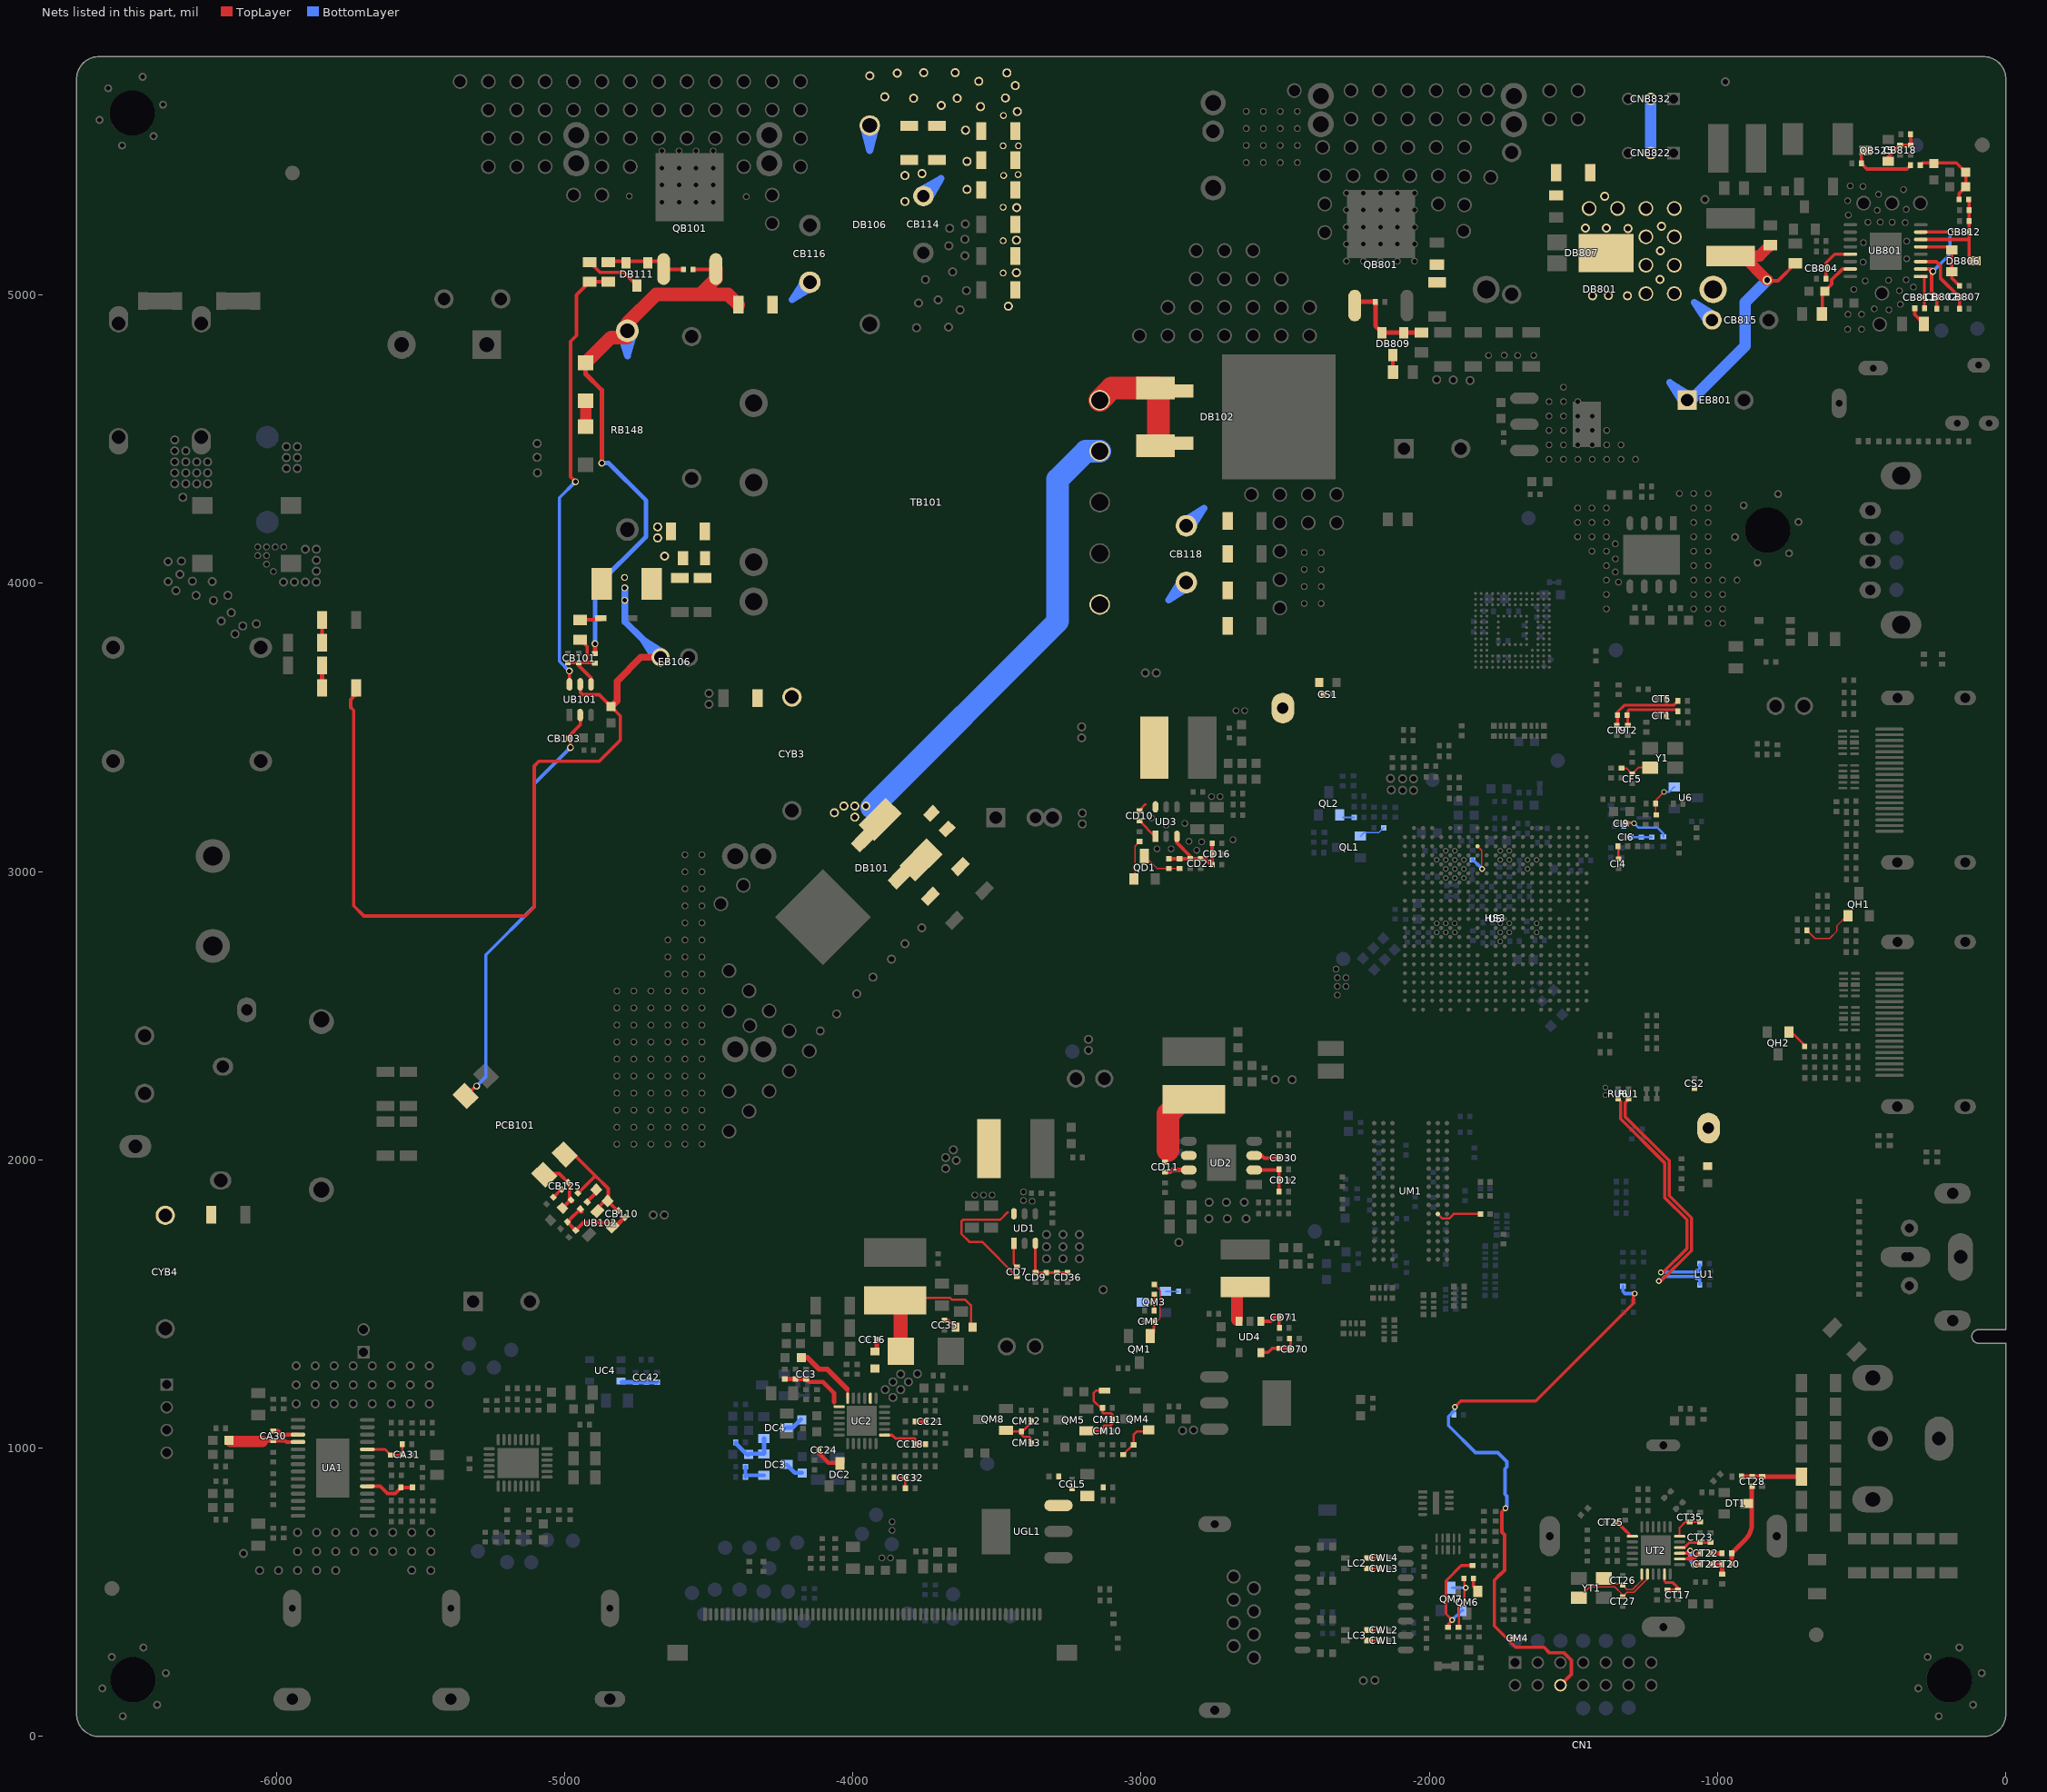
[diagram p0: the nets of this part, all layers, seen from the top]
# Altium PCB MISC84395.PcbDoc (part 21 of 26)
Units mil, origin at the board's own origin, x right, y up, seen from the top; angles counter-clockwise.
Board outline 6692.91 x 5826.77 mil, 2 copper layers (TopLayer, BottomLayer), stack 61.855 mil thick; 951 components, 565 nets, 4374 pads, 1804 vias.
Unrouted connection lines stored in the file: 1.

## Via types
v1: diameter 19.68, hole 11.81, TopLayer to BottomLayer, tented both sides, 1262 vias
v2: diameter 23.62, hole 15.75, TopLayer to BottomLayer, tented both sides, 524 vias
v3: diameter 31.5, hole 19.68, TopLayer to BottomLayer, tented both sides, 11 vias
v4: diameter 24, hole 16, TopLayer to BottomLayer, tented both sides, 6 vias
v5: diameter 19, hole 11.81, TopLayer to BottomLayer, tented both sides, 1 vias

## Nets (pads, with @x,y where several pads share a name; then routed paths per layer and width w, separated by ;. In a path a pad name is that pad's centre, name@x,y a point inside that pad or via, vN(x,y) a via of type N, cw(c..) or ccw(c..) an arc to the next point about the centre after c; other vN are vias at no path point) (continued)
NetCA30_1: CA30.1 LBA4.1 UA1.18 | length 232.8
  TopLayer w13: -6045.8,1026.21 CA30.1@-6010.6,1026.21 -5968.64,1026.21 -5963.94,1021.51 UA1.18@-5924.23,1021.51
  TopLayer w40: LBA4.1@-6157.49,1023.78 -6048.23,1023.78
NetCA30_2: CA30.2 UA1.17 | length 91.6
  TopLayer w13: CA30.2@-6010.6,1059.68 -5994.62,1059.68 -5982.04,1047.1 UA1.17@-5924.23,1047.1
NetCA31_1: CA31.1 RA11.2 RA21.2 UA1.10 | length 173.9
  TopLayer w8: UA1.10@-5684.07,995.92 -5622.59,995.92 RA11.2@-5602.61,975.94 -5558.43,975.94 -5563.33,980.83 RA21.2@-5563.33,1013.94
NetCB101_1: CB101.1 RB103.2 RB105.1 RB121.2 UB101.4 | length 287.9
  TopLayer w11.81: RB103.2@-4988.43,3724.09 CB101.1@-4950.43,3724.09 ; RB121.2@-4956.49,3804.11 -4945.3,3804.11 -4921.49,3780.3 -4921.49,3724.09 ; UB101.4@-4908.09,3649.3 -4908.09,3671.9 -4950.43,3714.24 CB101.1@-4950.43,3724.09 ; RB105.1@-4894.49,3722.83 -4895.74,3724.09 -4921.49,3724.09 ; CB101.1@-4950.43,3724.09 -4921.49,3724.09
NetCB102_1: CB102.1 DB104.K EB106.1 pad.VIA5@-4677,4157.3 pad.VIA5@-4677,4195.3 pad.VIA5@-4791,3941 pad.VIA5@-4791,3984 pad.VIA5@-4792,4020 RB102.1 RB116.1 UB101.5 | length 3115.5
  TopLayer w11.81: RB102.1@-5728.3,3631.59 RB102.1@-5722.89,3637 -5722.89,3610.72 -5726.65,3610.72 -5741.72,3595.65 -5741.72,3569.41 -5731.3,3559 -5731.3,2881.12 -5696.19,2846 -5135.76,2846 -5105.41,2876.35 -5105.41,3366.08 -5089,3382.49 -4879.3,3382.49 -4806.49,3455.3 -4806.49,3539.92 CB102.1@-4838.49,3571.92 -4879.87,3613.3 -4936.49,3613.3 -4945.49,3622.3 UB101.5@-4945.49,3649.3
  TopLayer w23.62: CB102.1@-4838.49,3571.92 -4817.8,3592.61 -4817.8,3660.2 -4735,3743 EB106.1@-4667,3743
  BottomLayer w23.62: pad.VIA5@-4791,3984 pad.VIA5@-4791,3941 -4791,3867 -4728.25,3804.25 EB106.1@-4667,3743
NetCB103_1: CB103.1 PCB101.4 UB101.2 | length 1493
  TopLayer w11.81: PCB101.4@-5342.71,2221.29 -5308,2256 v2(-5305,2256) ; v2(-4979.49,3430.3) -4979.49,3455.3 CB103.1@-4985.49,3461.3 -4985.49,3468.3 -4945.49,3508.3 UB101.2@-4945.49,3543
  BottomLayer w11.81: v2(-5305,2256) -5273.19,2287.81 -5273.19,2711.36 -5105.41,2879.15 -5105.41,3304.38 v2(-4979.49,3430.3)
NetCB109_1: CB109.1 CB110.1 PCB101.2 RB132.1 UB102.K | length 462.1
  TopLayer w11.81: PCB101.2@-4999.18,2019.18 -4968.18,2019.18 -4887,1938 ; RB132.1@-4953.34,1884.66 -4895,1943 -4895,1947 -4848,1900 -4848,1856 -4845.67,1853.67 CB109.1@-4839.67,1853.67 ; UB102.K@-4895,1823 -4860.33,1857.67 CB109.1@-4850.67,1857.67 ; CB109.1@-4845.67,1852.67 -4812.17,1819.17 CB110.1@-4808.17,1819.17
NetCB109_2: CB109.2 RB133.1 | length 55.6
  TopLayer w11.81: RB133.1@-4922.34,1854.66 CB109.2@-4883,1894
NetCB110_2: CB110.2 RB133.2 RB134.2 RB135.2 UB102.R | length 421.9
  TopLayer w11.81: -4980.17,1794.83 RB133.2@-4950,1825 ; RB133.2@-4945,1820 -4940,1825 -4940,1820 ; UB102.R@-4841.97,1769.97 -4835.04,1769.97 UB102.R@-4825.04,1769.97 ; UB102.R@-4823.04,1764.97 -4830.04,1764.97 UB102.R@-4825.04,1769.97 ; CB110.2@-4794.5,1800.5 UB102.R@-4825.04,1769.97 ; CB110.2@-4789.5,1800.5 -4820.04,1769.97 UB102.R@-4825.04,1769.97
  TopLayer w12: RB133.2@-4950,1825 RB135.2@-4990.17,1784.83 RB134.2@-4961.17,1755.83 -4935,1782 -4847.07,1782 UB102.R@-4835.04,1769.97 ; RB133.2@-4945,1820 -4940,1820
NetCB113_1: CB113.1 DB104.A pad.VIA5@-4653,4094.3 RB114.1 RB115.1
NetCB113_2: CB113.2 RB116.2
NetCB114_1: CB114.1@-3755,5343 pad.VIA5@-3760,5421 pad.VIA5@-3819,5324 pad.VIA5@-3819,5414 RB117.1 RB118.1
NetCB116_1: CB116.1 RB119.2
NetCB117_1: CB117.1 DB101.1 DB101.3 pad.VIA5@-3955,3227 pad.VIA5@-3993,3189 pad.VIA5@-3993,3227 pad.VIA5@-4031,3227 pad.VIA5@-4064,3204 TB101.7@-3143.53,3926.18 TB101.10 | length 1590.8
  BottomLayer w78.74: -3934.5,3222.5 -3289,3868 -3289,4360 -3191.32,4457.68 TB101.10@-3143.53,4457.68
NetCB117_2: CB117.2 RB128.1 RB129.1
NetCB118_1: CB118.1 DB102.1 DB102.3 TB101.11 | length 420.5
  TopLayer w78.74: TB101.11@-3143.53,4634.84 -3102.07,4676.3 -2940.17,4676.3 DB102.3@-2940.17,4476.3
NetCB118_2: CB118.2 RB124.1 RB125.1 RB126.1 RB136.1
NetCB125_1: CB125.1 PCB101.1 RB131.1 RB132.2 | length 212.2
  TopLayer w11.81: PCB101.1@-5072.89,1952.47 -5018.51,1952.47 -4983,1916.96 -4983,1865 RB132.2@-4979,1861 ; RB131.1@-5006.94,1833.06 RB132.2@-4979,1861 ; RB132.2@-4975,1857 RB132.2@-4974,1856 ; RB132.2@-4972,1856 RB132.2@-4974,1856 ; RB132.2@-4979,1861 RB132.2@-4974,1856
NetCB125_2: CB125.2 RB158.1 | length 39.4
  TopLayer w11.81: RB158.1@-5039.12,1869.99 CB125.2@-5011.24,1897.87
NetCB802_2: CB802.2 RB802.2 UB801.2 UB801.7 | length 441.7
  TopLayer w11.81: UB801.2@-295.53,5089.88 v2@-255.2,5089.88 ; UB801.7@-295.53,5217.83 -295.36,5218 v2(-194,5218) ; v2(-253.19,5081.87) -258,5077.05 -258,5010.59 CB802.2@-239.73,4992.32 RB802.2@-239.73,4952.32
  BottomLayer w11.81: v2(-253.19,5081.87) -194,5141.05 v2(-194,5218)
NetCB804_2: CB804.2 RB805.2 UB801.13 | length 150.5
  TopLayer w9.84: RB805.2@-624,5056 CB804.2@-624,5085.94 ; CB804.2@-620.03,5091.94 CB804.2@-624,5091.94 -624,5110.98 -593.92,5141.06 UB801.13@-539.63,5141.06 UB801.13@-540.17,5141.6
NetCB805_2: CB805.2 RB804.1 | length 67.2
  TopLayer w11.81: RB804.1@-316.2,4953.32 -316.2,4931.24 CB805.2@-284.27,4899.32
NetCB807_1: CB807.1 RB801.2 UB801.3 | length 250.5
  TopLayer w11.81: UB801.3@-295.53,5115.47 -241.47,5115.47 -227.47,5101.47 -227.47,5058.79 CB807.1@-161,4992.32 RB801.2@-161,4952.32
NetCB809_1: CB809.1 RB810.1
NetCB810_1: CB810.1 RB811.1
NetCB811_1: CB811.1 RB804.2 UB801.1 | length 123.8
  TopLayer w9.84: UB801.1@-295.53,5064.29 -282.73,5064.29 RB804.2@-282.73,4953.32
NetCB812_2: CB812.2 DB806.2 RB812.2 RB822.2 RB837.2 UB801.6 | length 382.6
  TopLayer w11.81: UB801.6@-295.53,5192.24 -128.71,5192.24 -127.95,5193 ; RB837.2@-127.95,5322.27 RB822.2@-127.95,5294.13 RB812.2@-127.95,5256.13 CB812.2@-127.95,5218 -127.95,5193 ; DB806.2@-109.97,5115 -127.95,5132.98 -127.95,5193
NetCB813_2: CB813.2 RB816.1 UB801.15 | length 212.9
  TopLayer w11.81: RB816.1@-644.19,4916.79 -637,4923.98 -637,4997 ; CB813.2@-628.19,5013 -604.24,5036.95 -604.24,5047 -604.24,5052.76 -567.12,5089.88 UB801.15@-539.63,5089.88
NetCB814_1: CB814.1 CB816.1 CB819.1 RB830.1 RB837.1 | length 279
  TopLayer w11.81: RB830.1@-297.27,5450 -289.27,5458 -172,5458 CB814.1@-139,5425 CB816.1@-139,5375 -162.46,5351.54 RB837.1@-162.46,5331
NetCB815_1: CB815.1 DB801.K DB807.2 EB801.1@-1105.65,4635 LB804.1 pad.VIA5@-828,5051 pad.VIA5@-1150.45,5004.44 pad.VIA5@-1150.45,5102.87 pad.VIA5@-1150.45,5201.29 pad.VIA5@-1150.45,5299.72 pad.VIA5@-1194.89,5238 pad.VIA5@-1198.89,5153 pad.VIA5@-1199.89,5054 pad.VIA5@-1248.88,5004.44 pad.VIA5@-1248.88,5102.87 pad.VIA5@-1248.88,5201.29 pad.VIA5@-1248.88,5299.72 pad.VIA5@-1310.89,5230 pad.VIA5@-1312.89,4997 pad.VIA5@-1347.3,5299.72 pad.VIA5@-1378.89,4998 pad.VIA5@-1385.89,5232 pad.VIA5@-1391.89,5342 pad.VIA5@-1433.89,4997 pad.VIA5@-1445.73,5299.72 pad.VIA5@-1458.89,5232 RB811.2 RB814.2 RB824.1 | length 984.6
  TopLayer w3: RB814.2@-747,5108 -745.09,5109.91 RB814.2@-730,5109.91
  TopLayer w11.81: pad.VIA5@-826.57,5049 -790.91,5049 RB814.2@-730,5109.91
  TopLayer w39.37: pad.VIA5@-828,5051 -912.04,5135.04 LB804.1@-955,5135.04 -854.87,5135.04 RB824.1@-823.45,5166.45
  BottomLayer w39.37: EB801.1@-1105.65,4635 -1092.65,4635 -905,4822.65 -905,4974 pad.VIA5@-828,5051
NetCB818_2: CB818.2 QB525.B RB833.1 RB834.2 | length 145.3
  TopLayer w11.81: QB525.B@-409,5463.5 -409,5477.66 -367.66,5519 CB818.2@-367,5519 RB833.1@-330,5519 RB834.2@-330,5554
NetCC3_1: CC3.1 RC7.1 RC9.1 UC2.1 | length 225.1
  TopLayer w15: RC9.1@-4236.24,1240.11 RC7.1@-4199.24,1240.11 CC3.1@-4162.24,1240.11 ; CC3.1@-4161.11,1240.11 CC3.1@-4162.24,1240.11 ; -4065.34,1159 -4065.34,1192.34 -4103,1230 -4152.13,1230 CC3.1@-4162.24,1240.11
NetCC11_1: CC11.1 UC2.24 | length 250.6
  TopLayer w10: -4019.61,1207.61 -4017.95,1205.95 UC2.24@-4017.95,1173.66
  TopLayer w18: CC11.1@-4179,1314 CC11.1@-4166.76,1314 ; CC11.1@-4178,1317 -4169.76,1317 CC11.1@-4166.76,1314 ; -4020.27,1205.95 -4088.32,1274 -4117.23,1274 -4157.23,1314 CC11.1@-4166.76,1314
NetCC16_2: CC16.2 RC11.1 | length 47
  TopLayer w15: RC11.1@-3923,1335.78 RC11.1@-3923,1341.52 ; RC11.1@-3917.26,1341.52 CC16.2@-3917.26,1377 CC16.2@-3917.26,1371.27
NetCC18_2: CC18.2 RC14.1 UC2.13 | length 165.5
  TopLayer w10: UC2.13@-3890,1045.71 -3863.71,1045.71 -3852.16,1034.16 -3787.16,1034.16 -3784.27,1031.27 CC18.2@-3784.27,1014 RC14.1@-3747.73,1014
NetCC21_1: CC21.1 RC13.2 | length 36.5
  TopLayer w10: RC13.2@-3784.26,1093 CC21.1@-3747.73,1093
NetCC24_2: CC24.2 DC2.2 | length 95.7
  TopLayer w15: CC24.2@-4117.57,994 -4117.57,982.57 -4084.5,949.5 -4050.47,949.5 DC2.2@-4048,947.03
NetCC27_1: CC27.1 DC3.2 | length 65.9
  BottomLayer w15: DC3.2@-4229.97,943.19 -4201.16,914.38 CC27.1@-4176,914.38
NetCC28_1: CC28.1 DC3.3 DC4.1 RC23.1 | length 170.9
  BottomLayer w15: RC23.1@-4405.73,1020.19 -4405.73,1017.28 -4366.65,978.19 CC28.1@-4361.19,978.19 -4358.69,980.69 DC3.3@-4308,980.69 DC4.1@-4308,1033.69
NetCC31_1: CC31.1 DC4.2 | length 62.3
  BottomLayer w15: DC4.2@-4229.97,1071.19 -4209.81,1071.19 CC31.1@-4180,1101
NetCC32_1: CC32.1 RC25.1 RC29.2 | length 74.5
  TopLayer w8: RC29.2@-3855.27,898 CC32.1@-3817.73,898 RC25.1@-3817.73,861
NetCC35_2: CC35.2 RC28.1 | length 48.1
  TopLayer w8: CC35.2@-3682,1443.74 -3667.52,1443.74 RC28.1@-3643.78,1420
NetCC42_1: CC42.1 RC31.2 RC35.1 UC4.3 | length 122.5
  BottomLayer w15: UC4.3@-4801.54,1229 RC35.1@-4753,1229 RC31.2@-4679,1229
NetCD7_1: CD7.1 UD1.1 | length 86.4
  TopLayer w8: UD1.1@-3441.4,1710.82 -3441.4,1639.13 CD7.1@-3431,1628.73
NetCD7_2: CD7.2 LD1.1 UD1.6 | length 471.5
  TopLayer w8: -3463,1818 -3489.12,1791.88 -3617.88,1791.88 -3623.46,1786.3 -3623.46,1743.59 -3595.63,1715.75 -3551.35,1715.75 -3431,1595.39 CD7.2@-3431,1595.26 ; UD1.6@-3442.58,1813.18 UD1.6@-3441.4,1813.18
NetCD9_1: CD9.1 CD36.1 RD1.1 RD4.2 UD1.3 | length 212.2
  TopLayer w10: CD9.1@-3366.6,1609.6 UD1.3@-3366.6,1710.82 ; CD9.1@-3366,1609 CD36.1@-3255,1609
NetCD10_1: CD10.1 UD3.1 | length 78
  TopLayer w8: CD10.1@-3005,3176.61 -3005,3175.19 -2951.82,3122.01 UD3.1@-2950.4,3122.01
NetCD10_2: CD10.2 LD3.1 UD3.6 | length 31.2
  TopLayer w8: CD10.2@-3005,3210.07 -3005,3213 -2985,3233
NetCD11_1: CD11.1 LD2.1 UD2.6 | length 197.2
  TopLayer w80: -2906.94,2034.06 -2906.94,2159.06 LD2.1@-2855.87,2210.13
NetCD11_2: CD11.2 UD2.7 | length 85.4
  TopLayer w15: CD11.2@-2917,1958.27 -2899,1958.27 -2892.27,1965 UD2.7@-2834.39,1965
NetCD12_1: CD12.1 RD7.1 RD12.1 UD2.2 | length 160.9
  TopLayer w12: UD2.2@-2607.61,1965 RD7.1@-2523.73,1965 ; RD12.1@-2521.73,1890 CD12.1@-2521.73,1929 RD7.1@-2521.73,1967
NetCD16_1: CD16.1 CD21.1 RD8.1 RD13.2 RD15.2 RD16.2 RD17.2 UD3.3 | length 328.2
  TopLayer w12: RD13.2@-2903.26,3044.57 RD17.2@-2866.26,3044.57 RD16.2@-2829.26,3044.57 ; UD3.3@-2875.6,3122.01 -2875.6,3099.6 -2829.26,3053.26 RD16.2@-2829.26,3044.57 ; RD16.2@-2829.26,3044.44 RD16.2@-2829.26,3044.57 ; CD21.1@-2793.39,3044.57 RD16.2@-2829.26,3044.57 ; CD21.1@-2793.26,3044.44 -2777.44,3044.44 -2757.19,3024.19 RD15.2@-2753.73,3024.19 RD8.1@-2753.73,3097.84
NetCD30_1: CD30.1 UD2.3 | length 89.6
  TopLayer w12: UD2.3@-2607.61,2015 -2582,2015 -2573,2006 CD30.1@-2521.73,2006
NetCD70_1: CD70.1 RD50.1 RD51.2 UD4.5 | length 141.3
  TopLayer w10: UD4.5@-2584.81,1332.15 -2559.85,1332.15 -2545.73,1346.27 RD51.2@-2520,1346.27 -2484.47,1346.27 -2481.73,1349.01 RD50.1@-2481.73,1380.26
NetCD71_2: CD71.2 RD3.1 UD4.1 | length 105.1
  TopLayer w12: UD4.1@-2584.81,1440.42 -2549.84,1440.42 -2536,1454.26 CD71.2@-2521.46,1454.26 RD3.1@-2521.46,1418.26
NetCF5_1: CF5.1 RF1.1 Y1.1 | length 116.5
  TopLayer w6: RF1.1@-1333.65,3358.47 -1316.65,3358.47 CF5.1@-1296.64,3338.47 -1274.38,3360.74 Y1.1@-1234.65,3360.74
NetCGL4_2: CGL4.2 CGL5.1 RG01.1 RG02.1 UGL1.3
NetCI4_2: CI4.2 RI4.1 | length 36.5
  TopLayer w8: CI4.2@-1343.65,3043.48 RI4.1@-1343.65,3080.01
NetCI6_1: CI6.1 RI7.1 RI9.1 | length 72.4
  BottomLayer w8: CI6.1@-1300.92,3119.74 -1264.91,3119.74 RI9.1@-1264.65,3119.47 RI7.1@-1228.65,3119.47
NetCI9_1: CI9.1 RI11.1 RI12.1 | length 184.1
  TopLayer w8: CI9.1@-1315.77,3167.74 v1(-1289.77,3167.74)
  BottomLayer w8: RI12.1@-1324.91,3159.74 -1316.91,3167.74 v1@-1297.65,3167.74 ; v1(-1289.77,3167.74) -1273.77,3151.74 -1208.26,3151.74 -1188.65,3132.13 RI11.1@-1188.65,3120.47
NetCM1_2: CM1.2 QM1.G RM5.2 | length 206.3
  TopLayer w5: CM1.2@-2955.26,1440 -2945,1440 -2935,1450 -2935,1548.73 RM5.2@-2954,1567.73
  TopLayer w8: QM1.G@-2968.6,1389.24 QM1.G@-2964.26,1393.58
  TopLayer w10: QM1.G@-2964.26,1393.58 -2955.26,1402.58 CM1.2@-2955.26,1440
NetCM4_2: CM4.2 CN1.6 RM13.1 RM14.1 | length 2204.5
  TopLayer w11.3: v1(-1912,1143) -1891.51,1163.49 -1631.53,1163.49 -1292.02,1503 v1@-1292.02,1532.42
  TopLayer w12: v1@-1739.17,788.57 -1748.29,779.45 -1748.29,708.71 -1739.17,699.59 -1739.17,576.69 -1753.58,562.28 -1754.72,562.28 -1774.75,542.25 -1774.75,383.85 -1700.3,309.39 -1602.21,309.39 -1583.21,290.39 -1532.75,290.39 -1507,264.64 -1507,216.28 CN1.6@-1545.28,178
  BottomLayer w12: v1(-1912,1143) -1912,1131.84 -1933.84,1110 -1933.84,1078.37 -1840.48,985 -1763,985 -1731.16,953.16 -1731.16,935.37 -1737.84,928.68 -1737.84,840.61 -1731.16,833.92 -1731.16,796.58 v1(-1735.88,791.85) ; RM13.1@-1328.77,1561.54 -1328.77,1543.77 -1321.61,1536.61 v1(-1287.83,1536.61)
NetCM10_2: CM10.2 CM11.1 DM1.K QM5.G RM12.2 | length 300.6
  TopLayer w8: CM10.2@-3133.73,1060 -3133.73,1072.27 -3127,1079 -3106,1079 -3100.27,1084.73 -3100.27,1117.43 -3104,1121.16 -3131.16,1121.16 -3133.73,1123.73 RM12.2@-3133.73,1140 -3140,1140 -3165,1165 -3165,1191 -3156,1200 DM1.K@-3127.15,1200
  TopLayer w10: QM5.G@-3189.16,1060 CM10.2@-3133.73,1060
NetCM12_1: CM12.1 CM13.2 QM8.G RM15.2 | length 167.5
  TopLayer w8: QM8.G@-3464.16,1058 RM15.2@-3414.73,1058 ; CM13.2@-3381.27,1017 -3381.27,1032.27 -3388,1039 -3407,1039 -3414.73,1046.73 RM15.2@-3414.73,1058 ; CM12.1@-3381.27,1095 -3381.27,1089.42 -3412.7,1058 RM15.2@-3414.73,1058
NetCNB822_2: CNB822.2 CNB832.2 | length 188.1
  BottomLayer w39.37: CNB832.2@-1232,5680 -1231.74,5679.74 CNB822.2@-1231.74,5492
NetCS1_1: CS1.1 HS3.1 RS1.2
NetCS2_1: CS2.1 HS3.2@-1031.98,2110.2 RS2.1
NetCT1_1: CT1.1 CT2.1 RT4.2 RT14.2 | length 250
  TopLayer w10: CT2.1@-1311.64,3506.47 -1311.65,3556.35 -1306.26,3561.74 -1143.2,3561.74 RT4.2@-1137.46,3556 ; CT1.1@-1177.43,3540 -1177.43,3561.32
NetCT5_2: CT5.2 CT9.1 RT2.2 RT14.1 | length 290.5
  TopLayer w10: CT9.1@-1347.38,3508.74 RT14.1@-1347.38,3542.74 -1347.38,3553.62 -1324.26,3576.74 -1153.12,3576.74 RT2.2@-1137.73,3592.13 ; -1177.26,3578 CT5.2@-1177.26,3598
NetCT17_2: CT17.2 RT1.1 UT2.23 | length 124.9
  TopLayer w10: UT2.23@-1184.36,563.58 -1184.36,539 -1179.26,533.9 -1155.15,533.9 -1138.21,516.96 CT17.2@-1138.21,507.93 ; RT1.1@-1174.21,507.92 CT17.2@-1138.21,507.93
NetCT20_1: CT20.1 CT28.1 DT1.2 LT6.2 | length 295.6
  TopLayer w15.8: CT20.1@-951.27,598.68 ccw(c-950.94,598.68) -951.17,598.45 LT6.2@-951.17,635.76 ccw(c-951.51,635.76) -951.27,636 -903.92,683.35 ccw(c-956.82,736.26) -882,736.26 CT28.1@-882,868.27
NetCT20_2: CT20.2 CT21.1 LT5.2 | length 74.8
  TopLayer w15.8: CT21.1@-1024.27,597.68 CT20.2@-984.74,597.69 -984,596.95 LT5.2@-984,562.74
NetCT21_2: CT21.2 UT2.3 | length 131.3
  TopLayer w10: UT2.3@-1113,635.63 UT2.3@-1132,635.63 -1104.37,635.63
  TopLayer w15.8: -1104.37,638.54 -1101.46,638.54 v1(-1095,645) ; v1(-1083,595) -1060.42,595 CT21.2@-1057.74,597.69
  BottomLayer w15.8: v1@-1095,641 -1095,626.97 ccw(c-1054.03,626.97) v1@-1083,598
NetCT22_1: CT22.1 LT6.1 | length 40
  TopLayer w15.8: CT22.1@-1024.68,635.76 LT6.1@-984.64,635.76
NetCT22_2: CT22.2 UT2.2 | length 77
  TopLayer w10: UT2.2@-1132,615.94 -1103.29,615.94
  TopLayer w15.8: -1100.39,617.73 -1096.96,617.73 ccw(c-1096.96,650.77) -1073.59,627.41 -1065.27,635.73 CT22.2@-1058.17,635.73
NetCT23_1: CT23.1 LT1.2 UT2.4 | length 120.1
  TopLayer w10: UT2.4@-1132,655.32 -1115.74,655.32 -1097.79,673.26 LT1.2@-1024.28,673.26 LT1.2@-1019.28,673.26
NetCT25_2: CT25.2 UT2.13 | length 80.7
  TopLayer w10: -1316.41,711.37 -1299.72,694.69 UT2.13@-1295.78,694.69
  TopLayer w12: CT25.2@-1355.27,746 -1351.03,746 -1316.41,711.37
NetCT26_2: CT26.2 UT2.19 YT1.1 | length 159.3
  TopLayer w5: YT1.1@-1378.29,529.31 CT26.2@-1330.28,529.31 ; CT26.2@-1329.28,529.31 CT26.2@-1329.28,525.26 -1314.02,510 -1295.19,510 -1263.1,542.09 UT2.19@-1263.1,563.58
NetCT27_2: CT27.2 UT2.20 YT1.3 | length 313.7
  TopLayer w5: YT1.3@-1481.31,481.54 -1443.53,519.31 -1357.31,519.31 -1329.29,491.29 CT27.2@-1329.29,484.74 -1314.03,500 -1291.05,500 -1243.42,547.63 UT2.20@-1243.42,563.58
NetCT28_2: CT28.2 CT60.2 DT4.K LT2.1 | length 209.9
  TopLayer w15.8: LT2.1@-917,901.15 -724.04,901.15 ccw(c-724.04,922.67) CT60.2@-708.82,907.46
NetCT35_1: CT35.1 RT6.1 UT2.6 | length 110.9
  TopLayer w5: RT6.1@-1061,744.27 -1059.91,744.27 RT6.1@-1059.12,743.49
  TopLayer w7: UT2.6@-1132,694.69 -1132,724 -1111.73,744.27 CT35.1@-1097,744.27 RT6.1@-1061,744.27
NetCWL1_2: CWL1.2 LC3.2 | length 37.4
  TopLayer w7: LC3.2@-2209.12,333 CWL1.2@-2171.74,333
NetCWL2_2: CWL2.2 LC3.3 | length 37.4
  TopLayer w7: LC3.3@-2209.13,369 CWL2.2@-2171.73,369
NetCWL3_2: CWL3.2 LC2.2 | length 41.7
  TopLayer w7: LC2.2@-2211.12,583 CWL3.2@-2173.73,583 ; LC2.2@-2201.24,582.88 LC2.2@-2196.88,582.88
NetCWL4_2: CWL4.2 LC2.3 | length 39
  TopLayer w7: LC2.3@-2210.35,620 CWL4.2@-2173.73,620 ; LC2.3@-2201.24,619.11 LC2.3@-2198.89,619.11
NetCYB3_1: CYB3.1 RB130.2
NetCYB4_1: CYB4.1 RB5.1
NetD4_K: D4.K R21.2 U6.2 | length 137.5
  TopLayer w6: R21.2@-1215.04,3197.01 D4.K@-1215.04,3235.74 ; D4.K@-1211.77,3235.74 D4.K@-1215.04,3235.74 ; v1(-1186,3276) -1200.68,3261.32 -1215.04,3246.96 D4.K@-1215.04,3235.74
  BottomLayer w6: v1(-1186,3276) -1167.5,3276 U6.2@-1150,3293.5
NetDB106_K: DB106.K pad.VIA5@-3557,5653 pad.VIA5@-3563,5741 pad.VIA5@-3604,5366 pad.VIA5@-3604,5463 pad.VIA5@-3609,5571 pad.VIA5@-3638,5682 pad.VIA5@-3645,5771 pad.VIA5@-3693,5657 pad.VIA5@-3754,5771 pad.VIA5@-3789,5682 pad.VIA5@-3846,5769 pad.VIA5@-3889,5687 pad.VIA5@-3941,5760 RB117.2 RB118.2 RB151.1 RB154.1 RB155.1
NetDB109_A: DB109.A QB101.S RB105.2 RB109.1 RB119.1 RB148.2 | length 2026.9
  TopLayer w11.81: RB109.1@-4554.54,5088 QB101.S@-4493.39,5088
  TopLayer w15.75: DB109.A@-4927,4764.74 -4927,4726 -4871,4670 v2(-4871,4417) ; RB105.2@-4894.49,3756.3 -4894,3756.79 v2(-4894,3790)
  TopLayer w47.24: DB109.A@-4927,4764.74 -4839.51,4852.23 -4782,4852.23 RB148.2@-4782,4875.23 -4782,4902 -4683,5001 -4432,5001 RB119.1@-4397,4966 ; -4530,5001 -4475.16,5055.84 QB101.S@-4475.16,5089.54
  BottomLayer w15.75: v2(-4894,3790) -4894,3985 -4717,4162 -4717,4287 -4847,4417 v2(-4871,4417)
NetDB109_K: DB109.K DB110.A | length 90.1
  TopLayer w39.37: DB110.A@-4927,4542.74 DB109.K@-4927,4632.85
NetDB111_1: DB111.1 DB111.3 QB101.G RB106.2 RB109.2 | length 280.5
  TopLayer w11.81: RB106.2@-4847.47,5117 QB101.G@-4656.26,5117 ; QB101.G@-4656.26,5065.98 QB101.G@-4656.26,5093.98 ; QB101.G@-4656.26,5066.09 QB101.G@-4656.15,5065.98 ; QB101.G@-4649.15,5088 RB109.2@-4588,5088
NetDB111_2: DB111.2 RB107.2 | length 197.3
  TopLayer w11.81: RB107.2@-4912.57,5113.87 -4876.7,5078 -4794.4,5078 DB111.2@-4748.97,5032.57
NetDB121_K: DB121.K RB121.1 | length 72.6
  TopLayer w11.81: RB121.1@-4946.39,3872.3 RB121.1@-4946.49,3872.39 -4945.88,3873 DB121.K@-4874.3,3873
NetDB806_1: DB806.1 DB806.3 RB827.2 UB801.5 | length 254
  TopLayer w11.81: UB801.5@-295.53,5166.65 -188,5166.65 -188,5058.32 RB827.2@-161,5031.32
NetDB809_1: DB809.1 DB809.3 QB801.G RB807.2 RB808.1 | length 316.7
  TopLayer w15.75: QB801.G@-2258.84,4963 QB801.G@-2255,4959.16 ; QB801.G@-2245.84,4976 RB808.1@-2187.2,4976 -2187.2,4892.2 DB809.3@-2164,4869 -2163.91,4869.09 RB807.2@-2028,4869.09
NetDB809_2: DB809.2 RB809.2 | length 59.2
  TopLayer w11.81: DB809.2@-2126.5,4790.97 -2126.5,4732.5 RB809.2@-2126,4732
NetDC1_A: DC1.A LC1.2 RC11.2 RC28.2 UC2.20 | length 468.1
  TopLayer w8: LC1.2@-3844.44,1521.69 -3662.67,1521.69 -3655.98,1515 -3609.95,1515 -3590.39,1495.44 -3590.39,1426.17 RC28.2@-3584.22,1420
  TopLayer w50: DC1.A@-3834.01,1352 LC1.2@-3834.01,1477.13
NetDC3_1: DC3.1 RC19.1 RC20.2 | length 102.5
  BottomLayer w12: RC20.2@-4372.27,936.19 RC19.1@-4372.27,900.19 -4366.77,905.69 DC3.1@-4308,905.69
NetLD5_1: LD5.1 UD4.3 | length 125.7
  TopLayer w40: UD4.3@-2667.21,1445.26 -2667.21,1531.09 LD5.1@-2639,1559.3
NetLU1_2: LU1.2 RU6.1 RU8.2 | length 896.3
  TopLayer w11: RU6.1@-1344.83,2210.23 -1336.83,2202.23 -1336.83,2142.66 -1184.34,1990.17 -1184.34,1869.37 -1107,1792.03 -1107,1692.49 -1189.6,1609.88 v1(-1196.74,1609.88)
  BottomLayer w11: v1(-1196.74,1609.88) -1195.86,1609 -1193.86,1611 -1080,1611 -1076.19,1614.81 LU1.2@-1067.65,1614.81 -1062.73,1619.73 RU8.2@-1062.73,1637
NetLU1_3: LU1.3 RU1.1 RU2.2 | length 940.3
  TopLayer w11: RU1.1@-1308.83,2210.23 -1320.83,2198.23 -1320.83,2149.28 -1168.34,1996.79 -1168.34,1876 -1091,1798.65 -1091,1685.86 v1@-1195.26,1581.61
  BottomLayer w11: v1(-1204,1580) -1197.86,1580 -1182.86,1595 -1080,1595 -1076.19,1591.19 LU1.3@-1067.65,1591.19 -1062.73,1586.27 RU2.2@-1062.73,1569
NetMR313_2: MR313.2 UM1.L8 | length 154.5
  TopLayer w7.87: UM1.L8@-1970.75,1812.46 -1955.01,1796.71 -1931.39,1796.71 -1915.64,1812.46 MR313.2@-1829.34,1812.46
NetQB525_C: QB525.C RB830.2 RB832.2 | length 235.3
  TopLayer w11.81: QB525.C@-487.03,5501.5 -501.27,5487.26 RB832.2@-501.27,5456 -482.11,5436.85 -343.89,5436.85 RB830.2@-330.73,5450
NetQD1_D: QD1.D RD13.1 RD17.1 | length 139.6
  TopLayer w5: QD1.D@-2988,3054.19 -2944.91,3011.1 RD13.1@-2903.26,3011.1 RD17.1@-2866.26,3011.1
NetQD1_G: QD1.G RD24.1 | length 138.6
  TopLayer w5: QD1.G@-3025.5,2974.19 -3021.25,2978.44 -3021.25,3088.02 RD24.1@-3005,3104.27
NetQH1_B: QH1.B RH3.1 | length 197.2
  TopLayer w5: RH3.1@-690.1,2796 -662.1,2768 -611.5,2768 -585.83,2793.67 -585.83,2812.63 -551.46,2847 QH1.B@-548.33,2847
NetQH2_B: QH2.B RH12.1 | length 74.2
  TopLayer w7: QH2.B@-752.5,2444.03 -744.73,2444.03 RH12.1@-697.73,2397.03
NetQL1_B: QL1.B RL7.1 | length 93
  BottomLayer w5: QL1.B@-2239,3122.5 -2226.84,3134.66 -2175.61,3134.66 RL7.1@-2158.27,3152
NetQL2_B: QL2.B RL9.1 | length 40.8
  BottomLayer w5: QL2.B@-2301.5,3188 RL9.1@-2260.73,3188
NetQM3_B: QM3.B RM7.2 | length 45
  BottomLayer w5: QM3.B@-2914.97,1544 RM7.2@-2870,1544
NetQM3_C: QM3.C RM1.1 RM5.1 | length 94.3
  TopLayer w5: RM1.1@-2954,1478 v1(-2954,1505) RM5.1@-2954,1534.27
  BottomLayer w5: QM3.C@-2992,1505 v1(-2954,1505)
NetQM4_B: QM4.B RM8.2 RM9.1 | length 144.8
  TopLayer w8: RM9.1@-3062,978.27 -3028.54,1011.73 RM8.2@-3026,1011.73 -3026,1046.75 -3015,1057.75 -2978.75,1057.75 QM4.B@-2973,1063.5
NetQM6_B: QM6.B RK7.1 | length 50.5
  TopLayer w10: RK7.1@-1847.27,548 -1847.27,519.77 QM6.B@-1831.5,504
NetQM7_B: QM7.B RK6.1 RK8.2 | length 343.2
  TopLayer w10: RK6.1@-1935,378.73 -1935,389 -1921,403 v1(-1921,404) -1942.5,425.5 -1942.5,540.07 -1889.3,593.27 RK8.2@-1850,593.27
  BottomLayer w10: v1(-1921,404) -1887,438 QM7.B@-1882.5,438
NetQM7_C: QM7.C RK3.1 RK7.2 | length 224.4
  TopLayer w8: RK3.1@-1898,378.73 -1898,449 -1879,468 -1879,546.27 RK7.2@-1880.73,548
  BottomLayer w8: QM7.C@-1920.5,516.03 v1@-1874.03,516.03
  other v1: -1874,516
NetR50_1: R50.1 U5.W13 | length 132.1
  TopLayer w3.94: v1@-1819,3008 v1@-1819,3009.31
  TopLayer w5: U5.W13@-1832.96,3088.05 -1818.37,3073.47 -1818.37,3009.94 v1@-1819,3009.31
  BottomLayer w12: R50.1@-1848.43,3040.54 v1(-1817.21,3009.31)
  BottomLayer w15: R50.1@-1850,3040.54 R50.1@-1848.43,3040.54
NetRA8_2: RA8.2 RA19.2 UA1.5 | length 175.7
  TopLayer w12: UA1.5@-5684.07,867.96 -5638.88,867.96 -5614.01,843.09 -5587.18,843.09 -5567.13,863.14 -5528.13,863.14 RA19.2@-5527.33,863.94
NetRB101_2: RB101.2 RB102.2 | length 78.1
  TopLayer w15.75: RB102.2@-5841,3637 -5840.83,3637.17 RB101.2@-5840.83,3715
NetRB106_1: RB106.1 RB107.1 UB101.6 | length 1533.4
  TopLayer w11.81: v2(-4983.49,3695.3) -4982.89,3694.7 UB101.6@-4982.89,3649.3 ; v2(-4962,4352) -4979.06,4369.06 -4979.06,4838.76 -4958.57,4859.25 -4958.57,4999.69 RB107.1@-4912.57,5045.68 RB106.1@-4847.47,5045.68
  BottomLayer w11.81: v2(-4983.49,3695.3) -5017.49,3729.3 -5017.49,4296.51 v2(-4962,4352)
NetRB141_1: RB141.1 RB142.2 | length 79.1
  TopLayer w11.81: RB141.1@-5841.21,3794 -5841,3794.21 RB142.2@-5841,3873
NetRB151_2: pad.VIA5@-3425.56,5517 pad.VIA5@-3426.56,5417 pad.VIA5@-3429.56,5636 pad.VIA5@-3431.56,5303 pad.VIA5@-3432.56,5077 pad.VIA5@-3432.56,5190 pad.VIA5@-3436.56,5726 pad.VIA5@-3460.56,4961 pad.VIA5@-3465.56,5770 pad.VIA5@-3470.56,5683 pad.VIA5@-3476.56,5414 pad.VIA5@-3477.56,5622 pad.VIA5@-3478.56,5076 pad.VIA5@-3478.56,5188 pad.VIA5@-3478.56,5304 pad.VIA5@-3478.56,5517 RB151.2 RB152.1 RB153.1 RB154.2 RB155.2 RB156.1